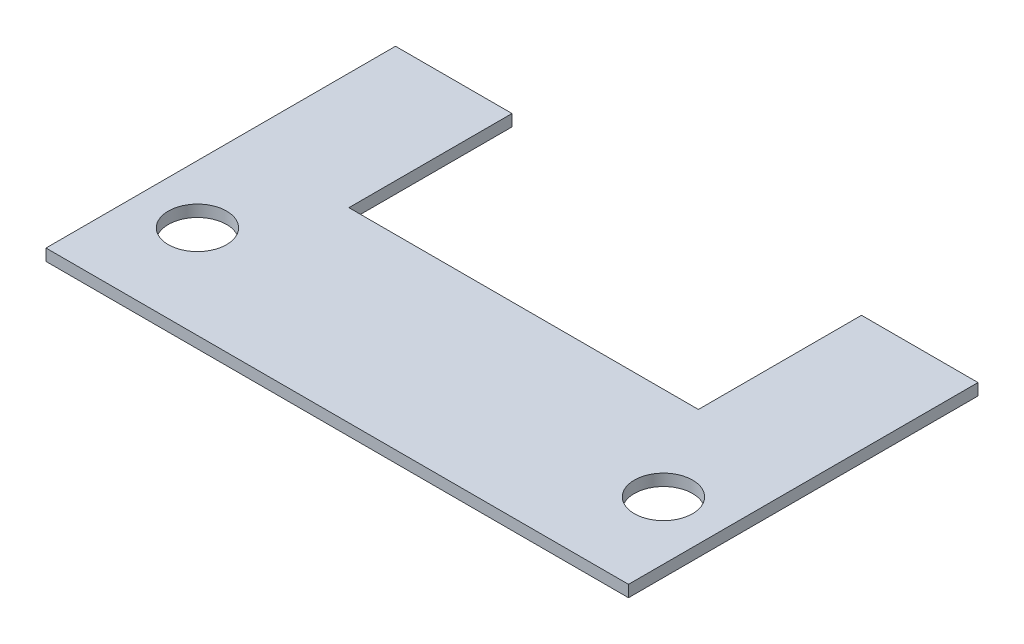
SolidWorks part; units mm, degrees
ref_plane "Front Plane" through (0, 0, 0) normal (0, 0, 1) x (1, 0, 0)
ref_plane "Top Plane" through (0, 0, 0) normal (0, 1, 0) x (1, 0, 0)
ref_plane "Right Plane" through (0, 0, 0) normal (1, 0, 0) x (0, 0, -1)
sketch "Sketch1" plane through (0, 0, 0) normal (0, 1, 0) x (1, 0, 0)
  line L0 (-12.5, 0) -> (12.5, 0)
  line L1 (12.5, 0) -> (12.5, 15)
  line L2 (12.5, 15) -> (7.5, 15)
  line L3 (7.5, 15) -> (7.5, 8)
  line L4 (7.5, 8) -> (-7.5, 8)
  line L5 (-12.5, 0) -> (-12.5, 15)
  line L6 (-12.5, 15) -> (-7.5, 15)
  line L7 (-7.5, 15) -> (-7.5, 8)
  circle A0 centre (10, 4) radius 1.25
  circle A1 centre (-10, 4) radius 1.25
  dimension "D6" = 2.5
  dimension "D7" = 20
  dimension "D1" = 25
  dimension "D2" = 5
  dimension "D3" = 5
  dimension "D4" = 15
  dimension "D5" = 8
  dimension "D8" = 10
  dimension "D9" = 4
extrude "Boss-Extrude1" add sketch "Sketch1" along normal blind 0.5
